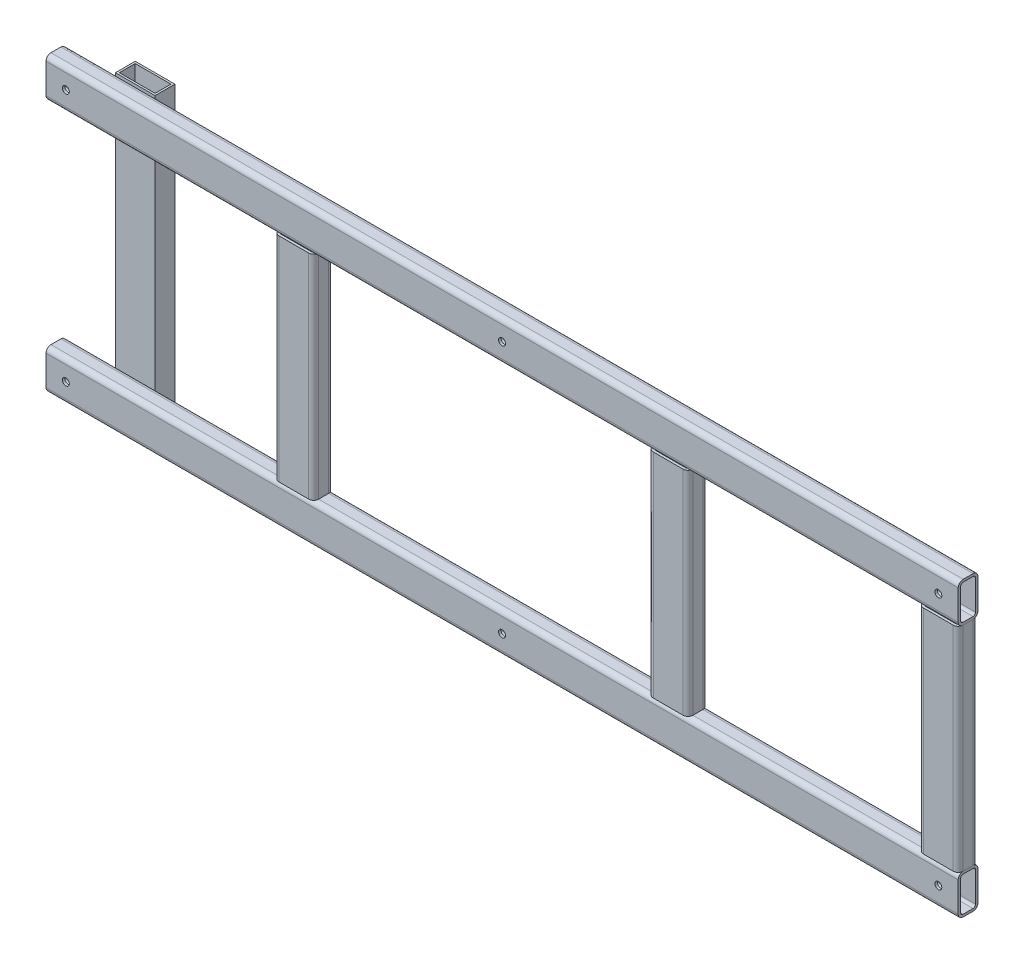
SolidWorks part; units mm, degrees
material "Q235"
ref_plane "Front Plane" through (0, 0, 0) normal (0, 0, 1) x (1, 0, 0)
ref_plane "Top Plane" through (0, 0, 0) normal (0, 1, 0) x (1, 0, 0)
ref_plane "Right Plane" through (0, 0, 0) normal (1, 0, 0) x (0, 0, -1)
sketch "草图1" plane through (0, 0, 0) normal (0, 0, 1) x (1, 0, 0)
  line L0 (0, 0) -> (900, 0)
  line L1 (900, 0) -> (900, -255)
  line L2 (900, -255) -> (0, -255)
  line L3 (0, -255) -> (0, 0)
  line L4 (250, 0) -> (250, -255)
  line L5 (627.4726, 0) -> (627.4726, -255)
  dimension "D1" = 255
  dimension "D2" = 900
  dimension "D3" = 650
other "Rect Tube 40X20X2.5(1)"
ref_plane "Plane1" through (0, 0, 0) normal (1, 0, 0) x (0, 0, 1)
sketch "Sketch1" plane through (0, 0, 0) normal (1, 0, 0) x (0, 0, 1)
  line L0 (-5, -17.5) -> (5, -17.5)
  line L1 (-7.5, -15) -> (-7.5, 15)
  line L2 (5, 17.5) -> (-5, 17.5)
  line L3 (7.5, 15) -> (7.5, -15)
  line L4 (-5, -20) -> (5, -20)
  line L5 (-10, -15) -> (-10, 15)
  line L6 (5, 20) -> (-5, 20)
  line L7 (10, 15) -> (10, -15)
  arc A0 (10, 15) -> (5, 20) centre (5, 15) ccw
  arc A1 (5, -20) -> (10, -15) centre (5, -15) ccw
  arc A2 (-10, -15) -> (-5, -20) centre (-5, -15) ccw
  arc A3 (-5, 20) -> (-10, 15) centre (-5, 15) ccw
  arc A4 (-5, 17.5) -> (-7.5, 15) centre (-5, 15) ccw
  arc A5 (7.5, 15) -> (5, 17.5) centre (5, 15) ccw
  arc A6 (5, -17.5) -> (7.5, -15) centre (5, -15) ccw
  arc A7 (-7.5, -15) -> (-5, -17.5) centre (-5, -15) ccw
  point P0 (0, 20)
  point P1 (10, 0)
  point P2 (0, -20)
  point P3 (-10, 0)
  point P4 (-10, 20)
  point P5 (10, 20)
  point P6 (10, -20)
  point P7 (-10, -20)
  point P8 (0, 0)
  point P33 (0, 0)
hole_wizard "M6 Clearance Hole1" positions "Sketch3" profile "Sketch4" hole size "M6" standard "GB"
sketch "Sketch3" plane through (0, 0, 10) normal (0, 0, 1) x (1, 0, 0)
  line L0 (0, 15) -> (0, -15) construction
  line L1 (920, 20) -> (0, 20) construction
  point P0 (20, -255)
  point P2 (20, 0)
  point P5 (460, 0)
  point P7 (460, -255)
  point P9 (900, 0)
  point P11 (900, -255)
  dimension "D1" = 255
  dimension "D2" = 440
  dimension "D3" = 440
  dimension "D4" = 20
  dimension "D5" = 20
sketch "Sketch4" plane through (20, -255, 10) normal (1, 0, 0) x (0, -1, 0)
  line L0 (0, 0) -> (0, 21.853)
  line L1 (0, 21.853) -> (3.5, 19.75)
  line L2 (3.5, 19.75) -> (3.5, 0)
  line L5 (3.5, 0) -> (0, 0)
  line L10 (0, 21.853) -> (-3.5, 19.75) construction
  line L11 (0, -6.35) -> (0, 107.95) construction
  dimension "孔直径" = 7
  dimension "孔深度" = 19.75
  dimension "导头角度" = 118
sketch "Sketch7" plane through (0, 0, -10) normal (0, 0, 1) x (1, 0, 0)
  line L0 (920, 20) -> (0, 20) construction
  line L4 (50, 20) -> (90, 20)
  line L5 (50, 20) -> (50, -275)
  line L6 (50, -275) -> (90, -275)
  line L7 (90, 20) -> (90, -275)
  line L8 (920, -275) -> (0, -275) construction
  line L9 (0, -15) -> (0, 15) construction
  dimension "D1" = 40
  dimension "D2" = 50
extrude "Boss-Extrude1" add sketch "Sketch7" against normal blind 20 separate body
sketch "Sketch8" plane through (0, 20, 0) normal (0, 1, 0) x (1, 0, 0)
  line L0 (88, 28) -> (52, 28)
  line L1 (52, 28) -> (52, 12)
  line L2 (52, 12) -> (88, 12)
  line L3 (88, 12) -> (88, 28)
  line L4 (50, 10) -> (90, 10)
  line L5 (90, 10) -> (90, 30)
  line L6 (90, 30) -> (50, 30)
  line L7 (50, 30) -> (50, 10)
  line L8 (50, 10) -> (90, 10) construction
  line L9 (90, 10) -> (90, 30) construction
  line L10 (90, 30) -> (50, 30) construction
  line L11 (50, 30) -> (50, 10) construction
  dimension "D1" = 0
  dimension "D2" = 2
extrude "Cut-Extrude1" cut sketch "Sketch8" against normal through all
equation "\"D1@Sketch1\" = \"Thickness@Sketch1\" * 2"
